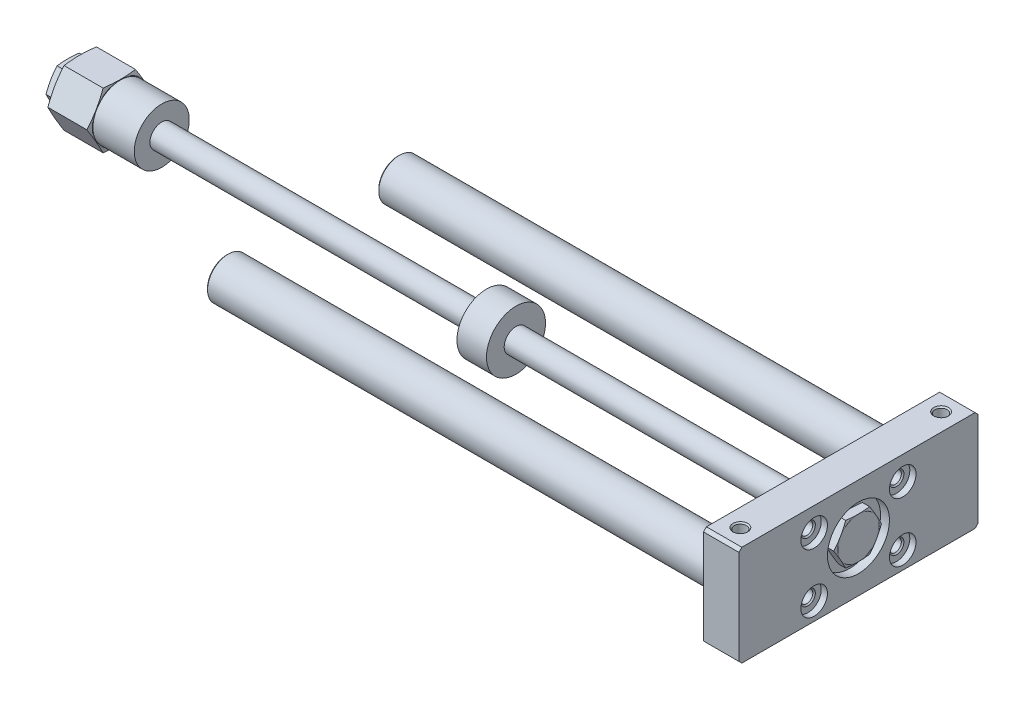
from build123d import *

# Parameters (mm, degrees)
BOSS_EXTRUDE1_DEPTH     = 12
CUT_EXTRUDE1_DEPTH      = 4
CUT_EXTRUDE1_DEPTH_BACK = 4
SKETCH9_W               = 28
SKETCH9_H               = 28
SKETCH10_W              = 3
SKETCH10_H              = 10.5
HOLE1_D                 = 4.134
HOLE1_DEPTH             = 12
HOLE1_CSINK_D           = 5
HOLE1_CSINK_ANGLE       = 90
HOLE1_TIP               = 1.193383006
HOLE2_D                 = 4.134
HOLE2_DEPTH             = 12
HOLE2_CSINK_D           = 5
HOLE2_CSINK_ANGLE       = 90
HOLE2_TIP               = 1.193383006
CUT_EXTRUDE2_DEPTH      = 3
CUT_EXTRUDE2_DEPTH_BACK = 3
SKETCH18_R              = 9.8
SKETCH21_W              = 38
SKETCH21_H              = 38
CUT_EXTRUDE3_DEPTH      = 14
SKETCH22_R              = 13
CUT_EXTRUDE4_DEPTH      = 4


with BuildPart() as part:
    # Sketch1 → Boss-Extrude1 (new body)
    with BuildSketch(Plane(origin=(14, 0, 0), x_dir=(0, 0, -1), z_dir=(1, 0, 0))):
        Polygon((-40.5, -16), (-39.5, -17), (39.5, -17), (40.5, -16), (40.5, 16), (39.5, 17), (-39.5, 17), (-40.5, 16), align=None)
    extrude(amount=-BOSS_EXTRUDE1_DEPTH)

    # Sketch2 → Revolve1 (revolve)
    with BuildSketch(Plane(origin=(0, -1.5, 0), x_dir=(1, 0, 0), z_dir=(0, 1, 0)), mode=Mode.PRIVATE) as revolve1_sk:
        Polygon((2, -29), (2, -36), (-170.5, -36), (-171, -35.5), (-171, -29), align=None)
    revolve(revolve1_sk.sketch.rotate(Axis((-171, -1.5, 29), (1, 0, 0)), 180), axis=Axis((-171, -1.5, 29), (1, 0, 0)))

    # Sketch3 → Revolve2 (revolve)
    with BuildSketch(Plane(origin=(0, -1.5, 0), x_dir=(1, 0, 0), z_dir=(0, 1, 0)), mode=Mode.PRIVATE) as revolve2_sk:
        Polygon((2, 29), (2, 22), (-170.5, 22), (-171, 22.5), (-171, 29), align=None)
    revolve(revolve2_sk.sketch.rotate(Axis((-171, -1.5, -29), (1, 0, 0)), 180), axis=Axis((-171, -1.5, -29), (1, 0, 0)))

    # Sketch4 → Cut-Revolve1 (revolve, cut)
    with BuildSketch(Plane(origin=(0, -11, 0), x_dir=(1, 0, 0), z_dir=(0, 1, 0)), mode=Mode.PRIVATE) as cut_revolve1_sk:
        Polygon((2, -15), (2, -12.5), (2.433, -12.933), (11.467, -12.933), (11.9, -12.5), (11.9, -10.5), (14, -10.5), (14, -15), align=None)
    revolve(cut_revolve1_sk.sketch.rotate(Axis((11.9, -11, 15), (-1, 0, 0)), 180), axis=Axis((11.9, -11, 15), (-1, 0, 0)), mode=Mode.SUBTRACT)

    # Sketch5 → Cut-Revolve2 (revolve, cut)
    with BuildSketch(Plane(origin=(0, -11, 0), x_dir=(1, 0, 0), z_dir=(0, 1, 0)), mode=Mode.PRIVATE) as cut_revolve2_sk:
        Polygon((2, 15), (2, 17.5), (2.433, 17.067), (11.467, 17.067), (11.9, 17.5), (11.9, 19.5), (14, 19.5), (14, 15), align=None)
    revolve(cut_revolve2_sk.sketch.rotate(Axis((11.9, -11, -15), (-1, 0, 0)), 180), axis=Axis((11.9, -11, -15), (-1, 0, 0)), mode=Mode.SUBTRACT)

    # Sketch6 → Cut-Revolve3 (revolve, cut)
    with BuildSketch(Plane(origin=(0, 9, 0), x_dir=(1, 0, 0), z_dir=(0, 1, 0)), mode=Mode.PRIVATE) as cut_revolve3_sk:
        Polygon((2, -15), (2, -12.5), (2.433, -12.933), (11.467, -12.933), (11.9, -12.5), (11.9, -10.5), (14, -10.5), (14, -15), align=None)
    revolve(cut_revolve3_sk.sketch.rotate(Axis((11.9, 9, 15), (-1, 0, 0)), 180), axis=Axis((11.9, 9, 15), (-1, 0, 0)), mode=Mode.SUBTRACT)

    # Sketch7 → Cut-Revolve4 (revolve, cut)
    with BuildSketch(Plane(origin=(0, 9, 0), x_dir=(1, 0, 0), z_dir=(0, 1, 0)), mode=Mode.PRIVATE) as cut_revolve4_sk:
        Polygon((2, 15), (2, 17.5), (2.433, 17.067), (11.467, 17.067), (11.9, 17.5), (11.9, 19.5), (14, 19.5), (14, 15), align=None)
    revolve(cut_revolve4_sk.sketch.rotate(Axis((11.9, 9, -15), (-1, 0, 0)), 180), axis=Axis((11.9, 9, -15), (-1, 0, 0)), mode=Mode.SUBTRACT)

    # Sketch8 → Revolve3 (revolve)
    with BuildSketch(Plane.XY, mode=Mode.PRIVATE) as revolve3_sk:
        Polygon((-112, 0), (-112, 10), (-102, 10), (-102, 4), (-2, 4), (-2, 7), (-1.624871131, 8.4), (1.624871131, 8.4), (2, 7), (2, 0), align=None)
    revolve(revolve3_sk.sketch.rotate(Axis((2, 0, 0), (-1, 0, 0)), 270), axis=Axis((2, 0, 0), (-1, 0, 0)))

    # Sketch9 → Cut-Extrude1 (cut, two sides: drawn at the far end of the back side and taken through both)
    with BuildSketch(Plane.ZY.offset(2).offset(-CUT_EXTRUDE1_DEPTH_BACK)):
        Rectangle(SKETCH9_W, SKETCH9_H)
        Polygon((4.041451884, -7), (8.082903769, 0), (4.041451884, 7), (-4.041451884, 7), (-8.082903769, 0), (-4.041451884, -7), align=None, mode=Mode.SUBTRACT)
    extrude(amount=CUT_EXTRUDE1_DEPTH + CUT_EXTRUDE1_DEPTH_BACK, mode=Mode.SUBTRACT)

    # Sketch10 → Cut-Revolve5 (revolve, cut)
    with BuildSketch(Plane.XY, mode=Mode.PRIVATE) as cut_revolve5_sk:
        with Locations((12.5, 5.25)):
            Rectangle(SKETCH10_W, SKETCH10_H)
    revolve(cut_revolve5_sk.sketch.rotate(Axis((14, 0, 0), (-1, 0, 0)), 270), axis=Axis((14, 0, 0), (-1, 0, 0)), mode=Mode.SUBTRACT)

    # Hole1
    with Locations(Plane(origin=(0, 17, 0), x_dir=(1, 0, 0), z_dir=(0, 1, 0))):
        with Locations((8, -34)):
            CounterSinkHole(HOLE1_D / 2, HOLE1_CSINK_D / 2, depth=HOLE1_DEPTH, counter_sink_angle=HOLE1_CSINK_ANGLE)
            with Locations((0, 0, -(HOLE1_DEPTH + HOLE1_TIP / 2))):  # 120° drill point
                Cone(0, HOLE1_D / 2, HOLE1_TIP, mode=Mode.SUBTRACT)

    # Hole2
    with Locations(Plane(origin=(0, 17, 0), x_dir=(1, 0, 0), z_dir=(0, 1, 0))):
        with Locations((8, 34)):
            CounterSinkHole(HOLE2_D / 2, HOLE2_CSINK_D / 2, depth=HOLE2_DEPTH, counter_sink_angle=HOLE2_CSINK_ANGLE)
            with Locations((0, 0, -(HOLE2_DEPTH + HOLE2_TIP / 2))):  # 120° drill point
                Cone(0, HOLE2_D / 2, HOLE2_TIP, mode=Mode.SUBTRACT)

    # Sketch16 → Cut-Revolve6 (revolve, cut)
    with BuildSketch(Plane(origin=(8, 0, 0), x_dir=(0, 0, -1), z_dir=(1, 0, 0)), mode=Mode.PRIVATE) as cut_revolve6_sk:
        Polygon((-9, -3.806616994), (-6.933, -5), (-6.933, -16.567), (-6.5, -17), (-9, -17), align=None)
    revolve(cut_revolve6_sk.sketch.rotate(Axis((8, -17, 9), (0, 1, 0)), 180), axis=Axis((8, -17, 9), (0, 1, 0)), mode=Mode.SUBTRACT)

    # Sketch17 → Cut-Revolve7 (revolve, cut)
    with BuildSketch(Plane(origin=(8, 0, 0), x_dir=(0, 0, -1), z_dir=(1, 0, 0)), mode=Mode.PRIVATE) as cut_revolve7_sk:
        Polygon((9, -3.806616994), (11.067, -5), (11.067, -16.567), (11.5, -17), (9, -17), align=None)
    revolve(cut_revolve7_sk.sketch.rotate(Axis((8, -17, -9), (0, 1, 0)), 180), axis=Axis((8, -17, -9), (0, 1, 0)), mode=Mode.SUBTRACT)

    # Sketch11 → Revolve4 (revolve)
    with BuildSketch(Plane.XY, mode=Mode.PRIVATE) as revolve4_sk:
        Polygon((11, 0), (11, 7), (11.375128869, 8.4), (13.624871131, 8.4), (14, 7), (14, 0), align=None)
    revolve(revolve4_sk.sketch.rotate(Axis((14, 0, 0), (-1, 0, 0)), 270), axis=Axis((14, 0, 0), (-1, 0, 0)))

    # Sketch18 → Cut-Extrude2 (cut, two sides: drawn at the far end of the back side and taken through both)
    with BuildSketch(Plane(origin=(14, 0, 0), x_dir=(0, 0, -1), z_dir=(1, 0, 0)).offset(-CUT_EXTRUDE2_DEPTH_BACK)):
        Circle(SKETCH18_R)
        Polygon((4.041451884, -7), (8.082903769, 0), (4.041451884, 7), (-4.041451884, 7), (-8.082903769, 0), (-4.041451884, -7), align=None, mode=Mode.SUBTRACT)
    extrude(amount=CUT_EXTRUDE2_DEPTH + CUT_EXTRUDE2_DEPTH_BACK, mode=Mode.SUBTRACT)

    # Sketch19 → Revolve5 (revolve)
    with BuildSketch(Plane.XY, mode=Mode.PRIVATE) as revolve5_sk:
        Polygon((-254, 0), (-254, 6.4), (-253.624871131, 7.8), (-250.375128869, 7.8), (-250, 6.4), (-250, 9.5), (-249.490896534, 11.4), (-236.509103466, 11.4), (-236, 9.5), (-236, 9.31), (-222, 9.31), (-222, 4), (-112, 4), (-112, 0), align=None)
    revolve(revolve5_sk.sketch.rotate(Axis((-112, 0, 0), (-1, 0, 0)), 270), axis=Axis((-112, 0, 0), (-1, 0, 0)))

    # Sketch20 → Revolve6 (revolve)
    with BuildSketch(Plane.XY, mode=Mode.PRIVATE) as revolve6_sk:
        Polygon((-256, 0), (-256, 3.233), (-255.233, 4), (-250, 4), (-250, 0), align=None)
    revolve(revolve6_sk.sketch.rotate(Axis((-250, 0, 0), (-1, 0, 0)), 270), axis=Axis((-250, 0, 0), (-1, 0, 0)))

    # Sketch21 → Cut-Extrude3 (cut)
    with BuildSketch(Plane.ZY.offset(250)):
        Rectangle(SKETCH21_W, SKETCH21_H)
        Polygon((5.484827557, -9.5), (10.969655115, 0), (5.484827557, 9.5), (-5.484827557, 9.5), (-10.969655115, 0), (-5.484827557, -9.5), align=None, mode=Mode.SUBTRACT)
    extrude(amount=-CUT_EXTRUDE3_DEPTH, mode=Mode.SUBTRACT)

    # Sketch22 → Cut-Extrude4 (cut)
    with BuildSketch(Plane.ZY.offset(254)):
        Circle(SKETCH22_R)
        Polygon((3.75277675, -6.5), (7.505553499, 0), (3.75277675, 6.5), (-3.75277675, 6.5), (-7.505553499, 0), (-3.75277675, -6.5), align=None, mode=Mode.SUBTRACT)
    extrude(amount=-CUT_EXTRUDE4_DEPTH, mode=Mode.SUBTRACT)


solid = part.part
